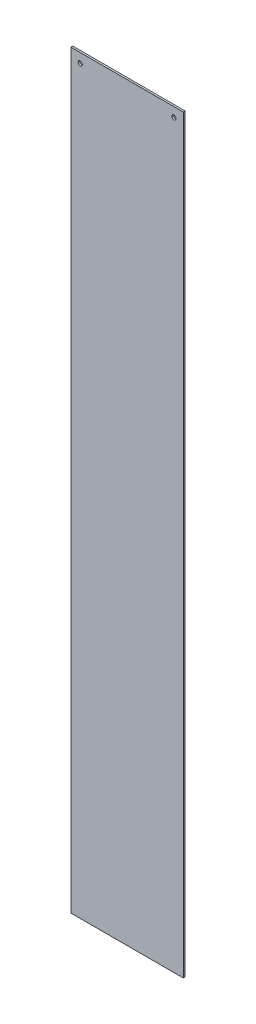
from build123d import *

# Parameters (mm, degrees)
SKETCH_1_W          = 120
SKETCH_1_H          = 800
EXTRUDE_1_DEPTH     = 2
SKETCH_2_R          = 2.25
CUT_EXTRUDE_1_DEPTH = 10


with BuildPart() as part:
    # 草图1 → 凸台-拉伸1 (new body)
    with BuildSketch(Plane.XY):
        Rectangle(SKETCH_1_W, SKETCH_1_H)
    extrude(amount=EXTRUDE_1_DEPTH)

    # 草图2 → 切除-拉伸1 (cut)
    with BuildSketch(Plane.XY.offset(2)):
        with Locations((-50, 390)):
            Circle(SKETCH_2_R)
        with Locations((50, 390)):
            Circle(SKETCH_2_R)
    extrude(amount=-CUT_EXTRUDE_1_DEPTH, mode=Mode.SUBTRACT)


solid = part.part
